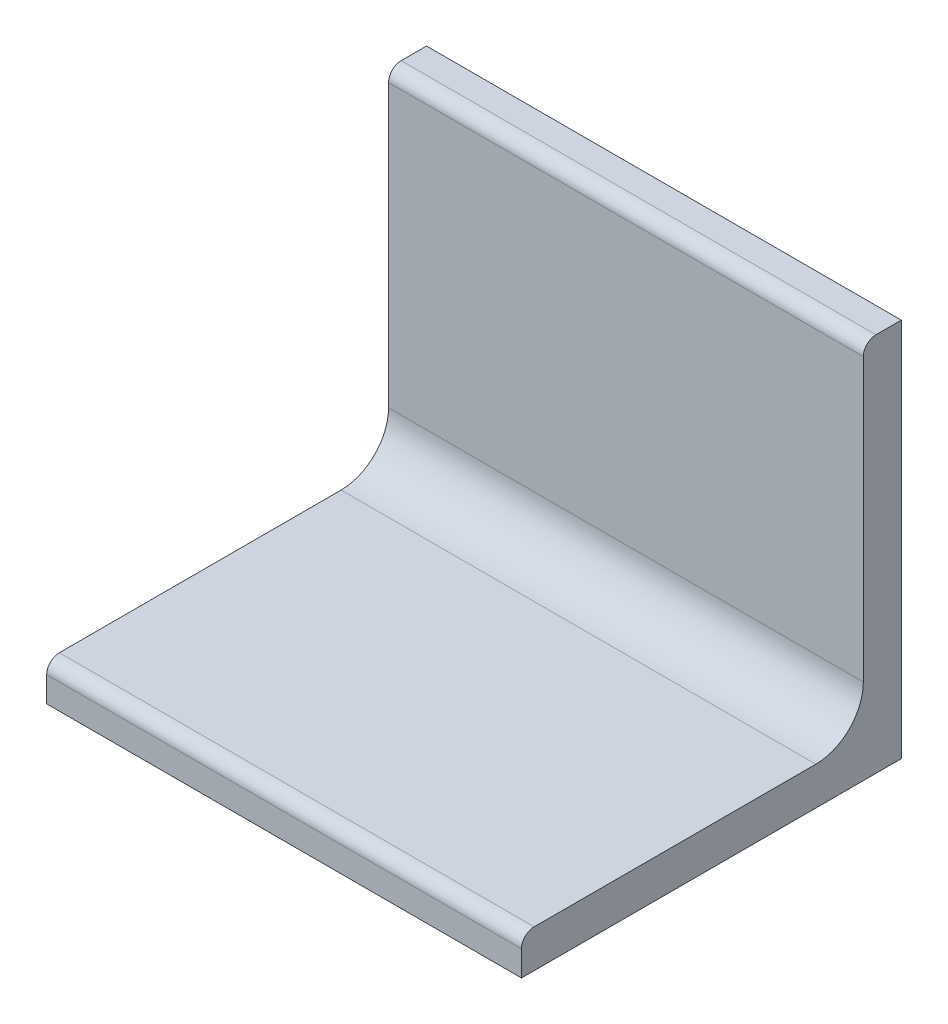
SolidWorks part; units mm, degrees
ref_plane "Front" through (0, 0, 0) normal (0, 0, 1) x (1, 0, 0)
ref_plane "Top" through (0, 0, 0) normal (0, 1, 0) x (1, 0, 0)
ref_plane "Right" through (0, 0, 0) normal (1, 0, 0) x (0, 0, -1)
other "Configuration Table"
sketch "Sketch1" plane through (0, 0, 0) normal (1, 0, 0) x (0, 1, 0)
  line L0 (0, 40) -> (0, 0)
  line L1 (0, 0) -> (40, 0)
  line L2 (4, 38.6667) -> (4, 9)
  line L3 (9, 4) -> (38.6667, 4)
  line L4 (0, 40) -> (2.6667, 40)
  line L5 (40, 0) -> (40, 2.6667)
  arc A0 (2.6667, 40) -> (4, 38.6667) centre (2.6667, 38.6667) cw
  arc A1 (40, 2.6667) -> (38.6667, 4) centre (38.6667, 2.6667) ccw
  arc A2 (4, 9) -> (9, 4) centre (9, 9) ccw
extrude "Base" add sketch "Sketch1" along normal blind 50
equation "\"r1@Sketch1\" = \"d@Sketch1\" / 3"
equation "\"d1@Sketch1\" = \"d@Sketch1\""
equation "\"b1@Sketch1\" = \"b@Sketch1\""
